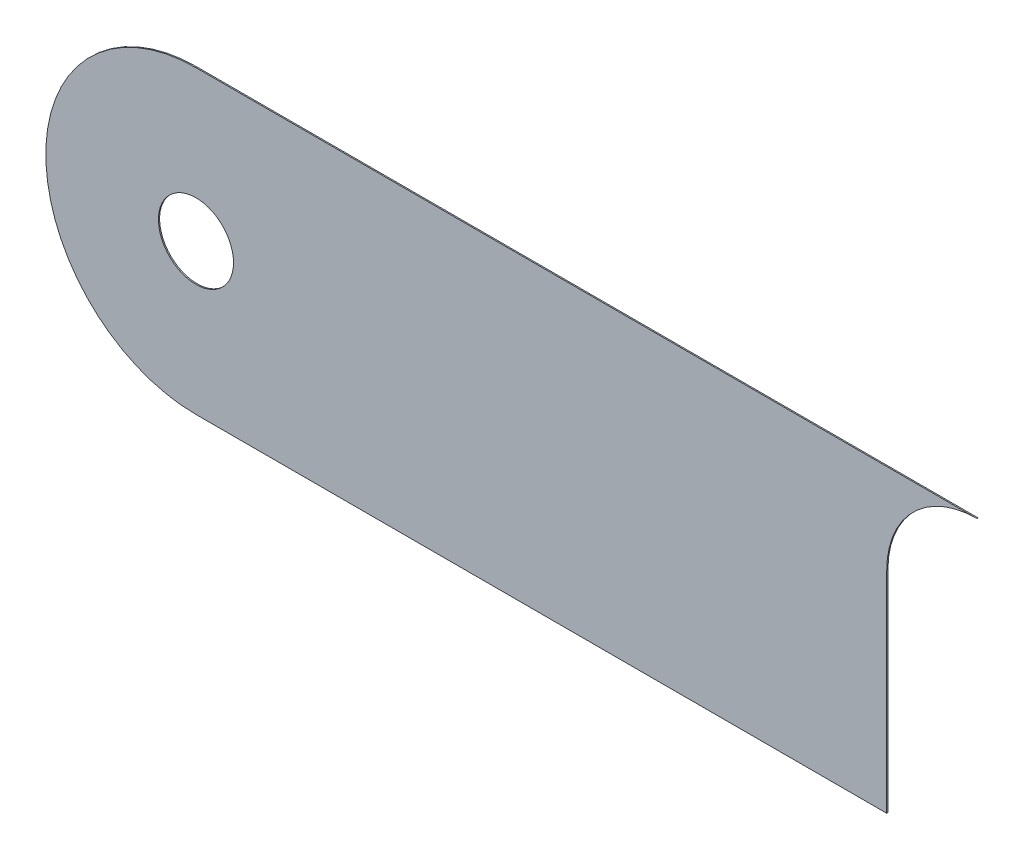
from build123d import *

# Parameters (mm, degrees)
SKETCH1_R           = 63.5
BOSS_EXTRUDE1_DEPTH = 1


with BuildPart() as part:
    # Sketch1 → Boss-Extrude1 (new, symmetric)
    with BuildSketch(Plane.XY):
        with BuildLine():
            Line((0, 254), (1320.8, 254))
            ThreePointArc((1320.8, 254), (1213.036926547, 209.363073453), (1168.4, 101.6))
            Line((1168.4, 101.6), (1168.4, -254))
            Line((1168.4, -254), (0, -254))
            ThreePointArc((0, -254), (-254, 0), (0, 254))
        make_face()
        Circle(SKETCH1_R, mode=Mode.SUBTRACT)
    extrude(amount=BOSS_EXTRUDE1_DEPTH, both=True)


solid = part.part
